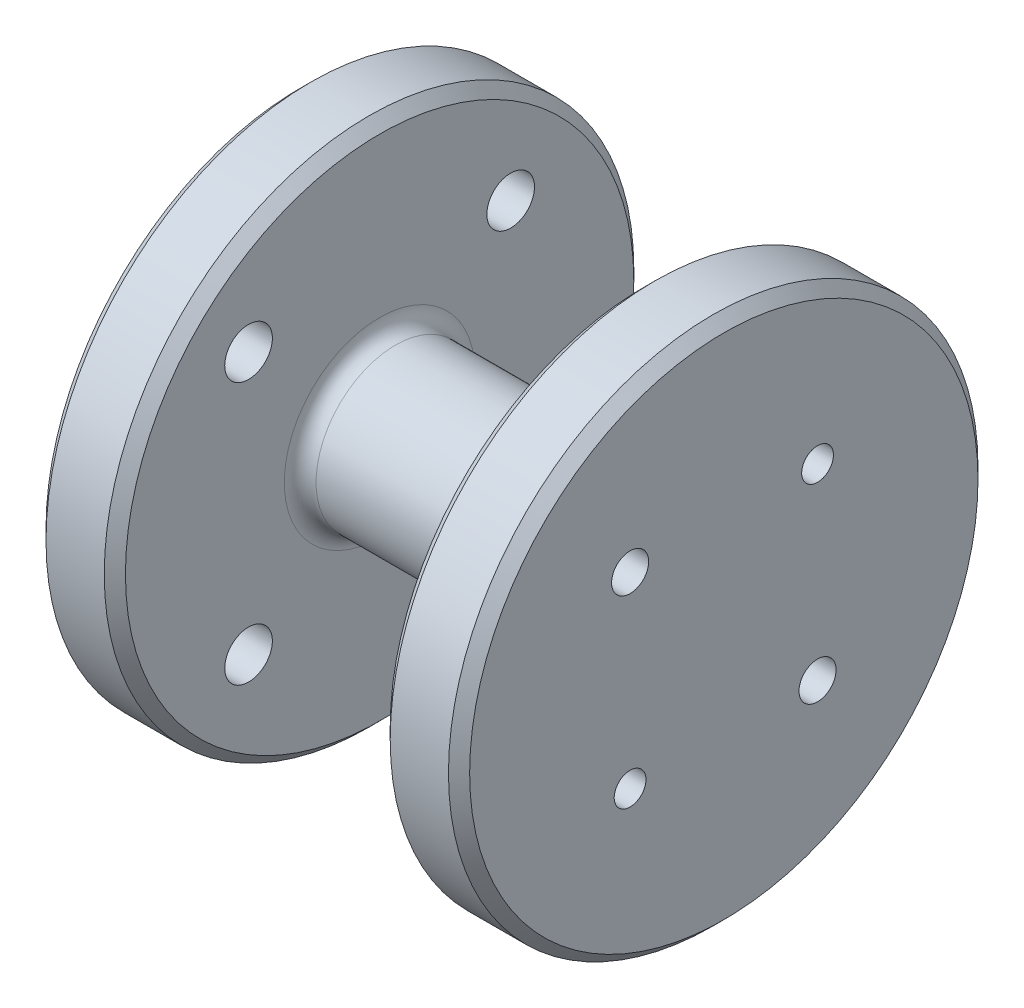
from build123d import *

# Parameters (mm, degrees)
SKETCH_1_R                = 50
EXTRUDE_1_DEPTH           = 15
SKETCH_2_R                = 15
EXTRUDE_2_DEPTH           = 50
SKETCH_3_R                = 50
EXTRUDE_3_DEPTH           = 15
HOLE_WIZARD_7_0_7_1_D     = 7
HOLE_WIZARD_7_0_7_1_DEPTH = 19.75
HOLE_WIZARD_7_0_7_1_TIP   = 2.103012167
MM_1_D                    = 6
MM_1_DEPTH                = 19.75
MM_1_TIP                  = 1.802581857
PATTERN_CIRCULAR_1_COUNT  = 4
FILLET_1_R                = 3
CHAMFER_1_SIZE            = 2


with BuildPart() as part:
    # 草图1 → 凸台-拉伸1 (new body)
    with BuildSketch(Plane(origin=(0, 0, 0), x_dir=(0, 0, -1), z_dir=(1, 0, 0))):
        Circle(SKETCH_1_R)
    extrude(amount=EXTRUDE_1_DEPTH)

    # 草图2 → 凸台-拉伸2 (add)
    with BuildSketch(Plane(origin=(15, 0, 0), x_dir=(0, 0, -1), z_dir=(1, 0, 0))):
        Circle(SKETCH_2_R)
    extrude(amount=EXTRUDE_2_DEPTH)

    # 草图3 → 凸台-拉伸3 (add)
    with BuildSketch(Plane(origin=(65, 0, 0), x_dir=(0, 0, -1), z_dir=(1, 0, 0))):
        Circle(SKETCH_3_R)
    extrude(amount=EXTRUDE_3_DEPTH)

    # Ø7.0 (7) 直径孔1
    with Locations(Plane(origin=(80, 0, 0), x_dir=(0, 0, -1), z_dir=(1, 0, 0))):
        with Locations((-17.698882733, 17.698882733), (17.698882733, -17.698882733)):
            Hole(HOLE_WIZARD_7_0_7_1_D / 2, depth=HOLE_WIZARD_7_0_7_1_DEPTH)
            with Locations((0, 0, -(HOLE_WIZARD_7_0_7_1_DEPTH + HOLE_WIZARD_7_0_7_1_TIP / 2))):  # 118° drill point
                Cone(0, HOLE_WIZARD_7_0_7_1_D / 2, HOLE_WIZARD_7_0_7_1_TIP, mode=Mode.SUBTRACT)

    # 大小mm 暗销孔1
    with Locations(Plane(origin=(80, 0, 0), x_dir=(0, 0, -1), z_dir=(1, 0, 0))):
        with Locations((-17.698882733, -17.698882733), (17.698882733, 17.698882733)):
            Hole(MM_1_D / 2, depth=MM_1_DEPTH)
            with Locations((0, 0, -(MM_1_DEPTH + MM_1_TIP / 2))):  # 118° drill point
                Cone(0, MM_1_D / 2, MM_1_TIP, mode=Mode.SUBTRACT)

    # 草图9 → Ø9.0 (9) 直径孔1 (revolve, cut)
    with BuildSketch(Plane(origin=(0, 24.748737342, -24.748737342), x_dir=(0, 0, 1), z_dir=(0, 1, 0))):
        Polygon((0, 0), (0, 22.453872786), (4.5, 19.75), (4.5, 0), align=None)
    hole_wizard_9_0_9_1 = revolve(axis=Axis((-6.35, 24.748737342, -24.748737342), (1, 0, 0)), mode=Mode.SUBTRACT)

    # 阵列(圆周)1: Ø9.0 (9) 直径孔1 ×4 about axis
    pattern_circular_1_axis = Axis((0, 0, 0), (1, 0, 0))
    for i in range(1, PATTERN_CIRCULAR_1_COUNT):
        add(hole_wizard_9_0_9_1.rotate(pattern_circular_1_axis, i * 360 / PATTERN_CIRCULAR_1_COUNT), mode=Mode.SUBTRACT)

    # 圆角1
    fillet_1_edges = [part.edges().sort_by_distance(p)[0] for p in [
        (15, 0, 15),
        (65, 0, 15),
    ]]
    fillet(fillet_1_edges, radius=FILLET_1_R)

    # 倒角1
    chamfer_1_edges = [part.edges().sort_by_distance(p)[0] for p in [
        (0, 0, 50),
        (15, 0, 50),
        (65, 0, 50),
        (80, 0, 50),
    ]]
    chamfer(chamfer_1_edges, length=CHAMFER_1_SIZE)


solid = part.part
